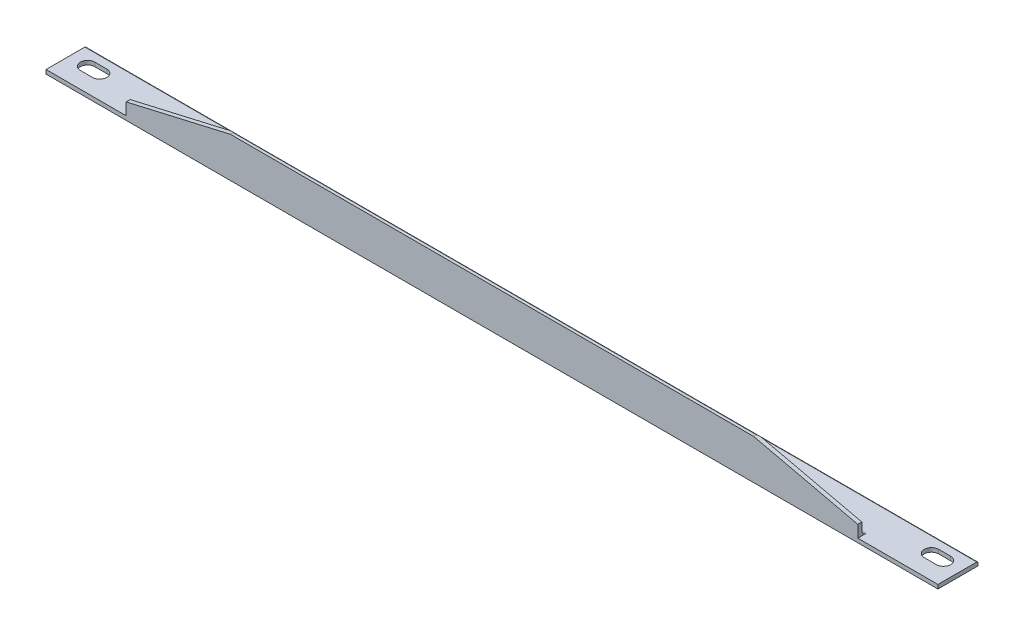
from build123d import *

# Parameters (mm, degrees)
HOT_ROLLED_EQUAL_LEG_ANGLE_STEEL_GB_T97_DEPTH = 1113
CUT_EXTRUDE1_REACH                            = 562.551
CUT_EXTRUDE2_REACH                            = 562.551
SKETCH16_W                                    = 100
SKETCH16_H                                    = 10.5
CUT_EXTRUDE3_DEPTH                            = 561.550845151
CUT_EXTRUDE3_DEPTH_BACK                       = 561.550845151


with BuildPart() as part:
    # Sketch11 → Hot-rolled equal-leg angle steel (gb t9787-1988) 50×5(1) (new body)
    with BuildSketch(Plane.YZ.offset(-556.5)):
        with BuildLine():
            Line((50, 0), (0, 0))
            Line((0, 0), (0, -50))
            Line((0, -50), (3.333333333, -50))
            ThreePointArc((3.333333333, -50), (4.511844635, -49.511844635), (5, -48.333333333))
            Line((5, -48.333333333), (5, -10.5))
            ThreePointArc((5, -10.5), (6.610912703, -6.610912703), (10.5, -5))
            Line((10.5, -5), (48.333333333, -5))
            ThreePointArc((48.333333333, -5), (49.511844635, -4.511844635), (50, -3.333333333))
            Line((50, -3.333333333), (50, 0))
        make_face()
    extrude(amount=HOT_ROLLED_EQUAL_LEG_ANGLE_STEEL_GB_T97_DEPTH)

    # Sketch13 → Cut-Extrude1 (cut, up to next)
    with BuildSketch(Plane(origin=(0, 5, 0), x_dir=(1, 0, 0), z_dir=(0, 1, 0)), mode=Mode.PRIVATE) as cut_extrude1_sk1:
        with BuildLine():
            Line((-534, 38.416666667), (-519, 38.416666667))
            ThreePointArc((-519, 38.416666667), (-510, 29.416666667), (-519, 20.416666667))
            Line((-519, 20.416666667), (-534, 20.416666667))
            ThreePointArc((-534, 20.416666667), (-543, 29.416666667), (-534, 38.416666667))
        make_face()
    cut_extrude1_tool1 = extrude(cut_extrude1_sk1.sketch, amount=-CUT_EXTRUDE1_REACH, mode=Mode.PRIVATE) & part.part
    # Sketch13 → Cut-Extrude1 (cut, up to next)
    with BuildSketch(Plane(origin=(0, 5, 0), x_dir=(1, 0, 0), z_dir=(0, 1, 0)), mode=Mode.PRIVATE) as cut_extrude1_sk2:
        with BuildLine():
            Line((534, 20.416666667), (519, 20.416666667))
            ThreePointArc((519, 20.416666667), (510, 29.416666667), (519, 38.416666667))
            Line((519, 38.416666667), (534, 38.416666667))
            ThreePointArc((534, 38.416666667), (543, 29.416666667), (534, 20.416666667))
        make_face()
    cut_extrude1_tool2 = extrude(cut_extrude1_sk2.sketch, amount=-CUT_EXTRUDE1_REACH, mode=Mode.PRIVATE) & part.part
    add(cut_extrude1_tool1.solids().sort_by_distance((-526.5, 5, -29.416667))[0], mode=Mode.SUBTRACT)
    add(cut_extrude1_tool2.solids().sort_by_distance((526.5, 5, -29.416667))[0], mode=Mode.SUBTRACT)

    # Sketch16 → Cut-Extrude2 (cut, up to next)
    with BuildSketch(Plane(origin=(0, 5, 0), x_dir=(1, 0, 0), z_dir=(0, 1, 0)), mode=Mode.PRIVATE) as cut_extrude2_sk1:
        with Locations((506.5, 5.25)):
            Rectangle(SKETCH16_W, SKETCH16_H)
    cut_extrude2_tool1 = extrude(cut_extrude2_sk1.sketch, amount=CUT_EXTRUDE2_REACH, mode=Mode.PRIVATE) & part.part
    # Sketch16 → Cut-Extrude2 (cut, up to next)
    with BuildSketch(Plane(origin=(0, 5, 0), x_dir=(1, 0, 0), z_dir=(0, 1, 0)), mode=Mode.PRIVATE) as cut_extrude2_sk2:
        with Locations((-506.5, 5.25)):
            Rectangle(SKETCH16_W, SKETCH16_H)
    cut_extrude2_tool2 = extrude(cut_extrude2_sk2.sketch, amount=CUT_EXTRUDE2_REACH, mode=Mode.PRIVATE) & part.part
    add(cut_extrude2_tool1.solids().sort_by_distance((506.5, 5, -5.25))[0], mode=Mode.SUBTRACT)
    add(cut_extrude2_tool2.solids().sort_by_distance((-506.5, 5, -5.25))[0], mode=Mode.SUBTRACT)

    # Sketch17 → Cut-Extrude3 (cut, two sides: drawn at the far end of the back side and taken through both)
    with BuildSketch(Plane(origin=(0, 0, -5), x_dir=(-1, 0, 0), z_dir=(0, 0, -1)).offset(-CUT_EXTRUDE3_DEPTH_BACK)):
        Polygon((326.5, 50), (456.5, 50), (456.5, 20), align=None)
        Polygon((-456.5, 20), (-326.5, 50), (-456.5, 50), align=None)
    extrude(amount=CUT_EXTRUDE3_DEPTH + CUT_EXTRUDE3_DEPTH_BACK, mode=Mode.SUBTRACT)


solid = part.part
